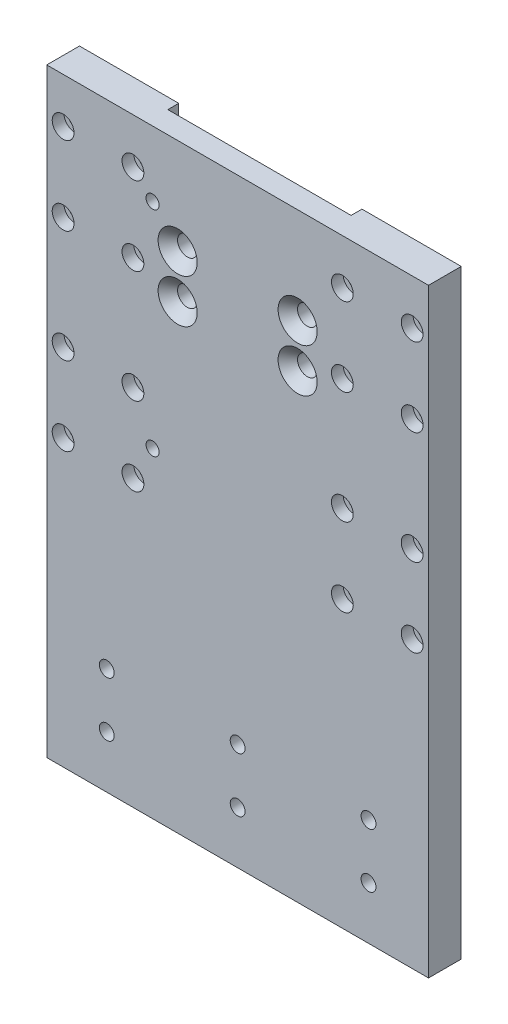
SolidWorks part; units mm, degrees
material "6061Al"
ref_plane "前视基准面" through (0, 0, 0) normal (0, 0, 1) x (1, 0, 0)
ref_plane "上视基准面" through (0, 0, 0) normal (0, 1, 0) x (1, 0, 0)
ref_plane "右视基准面" through (0, 0, 0) normal (1, 0, 0) x (0, 0, -1)
sketch "草图1" plane through (0, 0, 0) normal (0, 0, 1) x (1, 0, 0)
  line L1 (-87.5, -137.5) -> (87.5, -137.5)
  line L2 (-87.5, -137.5) -> (-87.5, 137.5)
  line L3 (-87.5, 137.5) -> (87.5, 137.5)
  line L4 (87.5, -137.5) -> (87.5, 137.5)
  line L5 (-87.5, -137.5) -> (87.5, 137.5) construction
  line L6 (-87.5, 137.5) -> (87.5, -137.5) construction
  point P0 (0, 0)
  dimension "D1" = 175
  dimension "D2" = 275
extrude "凸台-拉伸1" add sketch "草图1" along normal blind 10
sketch "草图10" plane through (0, 0, 0) normal (0, 0, -1) x (-1, 0, 0)
  line L0 (87.5, -137.5) -> (-87.5, -137.5) construction
  line L1 (-87.5, 137.5) -> (-42, 137.5)
  line L2 (-87.5, 137.5) -> (-87.5, -137.5)
  line L3 (-87.5, -137.5) -> (-42, -137.5)
  line L4 (-42, 137.5) -> (-42, -137.5)
  line L5 (0, 0) -> (0, 210.5491) construction
  line L6 (42, 137.5) -> (42, -137.5)
  line L7 (87.5, -137.5) -> (42, -137.5)
  line L8 (87.5, 137.5) -> (87.5, -137.5)
  line L9 (87.5, 137.5) -> (42, 137.5)
  dimension "D1" = 45.5
extrude "凸台-拉伸2" add sketch "草图10" along normal blind 5
hole_wizard "M8 六角凹锥坑螺钉的锥形沉头孔1" positions "草图2" profile "草图3" countersink size "M8" standard "ISO" end condition through all
sketch "草图2" plane through (0, 0, 10) normal (0, 0, 1) x (1, 0, 0)
  point P0 (-27.5, 93.5)
  point P3 (-27.5, 73.5)
  point P6 (27.5, 93.5)
  point P9 (27.5, 73.5)
sketch "草图3" plane through (-27.5, 93.5, 10) normal (1, 0, 0) x (0, -1, 0)
  line L0 (0, 0) -> (0, 15)
  line L1 (0, 15) -> (4.5, 15)
  line L2 (4.5, 15) -> (4.5, 4.46)
  line L3 (4.5, 4.46) -> (8.96, 0)
  line L5 (8.96, 0) -> (0, 0)
  line L6 (-4.5, 4.46) -> (-8.96, 0) construction
  line L11 (0, -6.35) -> (0, 107.95) construction
  dimension "通孔孔直径" = 9
  dimension "通孔孔深度" = 15
  dimension "近端锥形沉头孔直径" = 17.92
  dimension "近端锥形沉头孔角度" = 90
hole_wizard "M8 螺纹孔1" positions "草图4" profile "草图5" tap size "M8" standard "ISO" end condition through all
sketch "草图4" plane through (0, 0, 10) normal (0, 0, 1) x (1, 0, 0)
  line L0 (0, 0) -> (0, -137.5) construction
  line L1 (-87.5, -137.5) -> (87.5, -137.5) construction
  line L3 (60, -113.5) -> (60, -88.5) construction
  point P0 (0, -113.5)
  point P2 (-60, -113.5)
  point P4 (60, -113.5)
  point P19 (0, -88.5)
  point P20 (-60, -88.5)
  point P21 (60, -88.5)
  dimension "D1" = 120
  dimension "D2" = 24
  dimension "D4" = 25
  dimension "D3" = 2
sketch "草图5" plane through (0, -113.5, 10) normal (1, 0, 0) x (0, -1, 0)
  line L0 (0, 0) -> (0, 15)
  line L1 (0, 15) -> (3.4, 15)
  line L2 (3.4, 15) -> (3.4, 0)
  line L5 (3.4, 0) -> (0, 0)
  line L11 (0, -6.35) -> (0, 107.95) construction
  dimension "通孔螺纹孔钻头直径" = 6.8
  dimension "通孔螺纹孔钻头深度" = 15
cosmetic thread "孔螺蚊线1" parameters "D2"=8
cosmetic thread "孔螺蚊线2" parameters "D2"=8
cosmetic thread "孔螺蚊线3" parameters "D2"=8
cosmetic thread "孔螺蚊线4" parameters "D2"=8
cosmetic thread "孔螺蚊线5" parameters "D2"=8
cosmetic thread "孔螺蚊线6" parameters "D2"=8
hole_wizard "M5 六角凹头螺钉的柱形沉头孔1" positions "草图6" profile "草图7" counterbore size "M5" standard "ISO" end condition through all
sketch "草图6" plane through (0, 0, 10) normal (0, 0, 1) x (1, 0, 0)
  line L0 (0, 0) -> (0, 187.0882) construction
  point P0 (-80, 116.75)
  point P3 (-48, 116.75)
  point P6 (-80, 80.75)
  point P9 (-48, 80.75)
  point P12 (-80, 29.25)
  point P15 (-48, 29.25)
  point P18 (-80, -6.75)
  point P21 (-48, -6.75)
  point P29 (48, -6.75)
  point P30 (80, -6.75)
  point P31 (48, 29.25)
  point P32 (80, 29.25)
  point P33 (48, 80.75)
  point P34 (80, 80.75)
  point P35 (48, 116.75)
  point P36 (80, 116.75)
sketch "草图7" plane through (-80, 116.75, 10) normal (1, 0, 0) x (0, -1, 0)
  line L0 (0, 0) -> (0, 15)
  line L1 (0, 15) -> (2.75, 15)
  line L3 (2.75, 15) -> (2.75, 5.4)
  line L4 (2.75, 5.4) -> (5, 5.4)
  line L5 (5, 5.4) -> (5, 0)
  line L7 (5, 0) -> (0, 0)
  line L11 (0, -6.35) -> (0, 107.95) construction
  dimension "通孔孔直径" = 5.5
  dimension "通孔孔深度" = 15
  dimension "柱形沉头孔直径" = 10
  dimension "柱形沉头孔深度" = 5.4
hole_wizard "Ø6.0mm 暗销孔1" positions "草图8" profile "草图9" hole size "Ø6.0" standard "ISO" end condition through all
sketch "草图8" plane through (0, 0, 10) normal (0, 0, 1) x (1, 0, 0)
  line L0 (-87.5, 137.5) -> (-87.5, -137.5) construction
  line L1 (87.5, 137.5) -> (-87.5, 137.5) construction
  point P0 (-39, 107.5)
  point P2 (-39, 9.5)
  dimension "D1" = 48.5
  dimension "D2" = 30
  dimension "D3" = 98
sketch "草图9" plane through (-39, 107.5, 10) normal (1, 0, 0) x (0, -1, 0)
  line L0 (0, 0) -> (0, 15)
  line L1 (0, 15) -> (3, 15)
  line L2 (3, 15) -> (3, 0)
  line L5 (3, 0) -> (0, 0)
  line L11 (0, -6.35) -> (0, 107.95) construction
  dimension "通孔孔直径" = 6
  dimension "通孔孔深度" = 15
